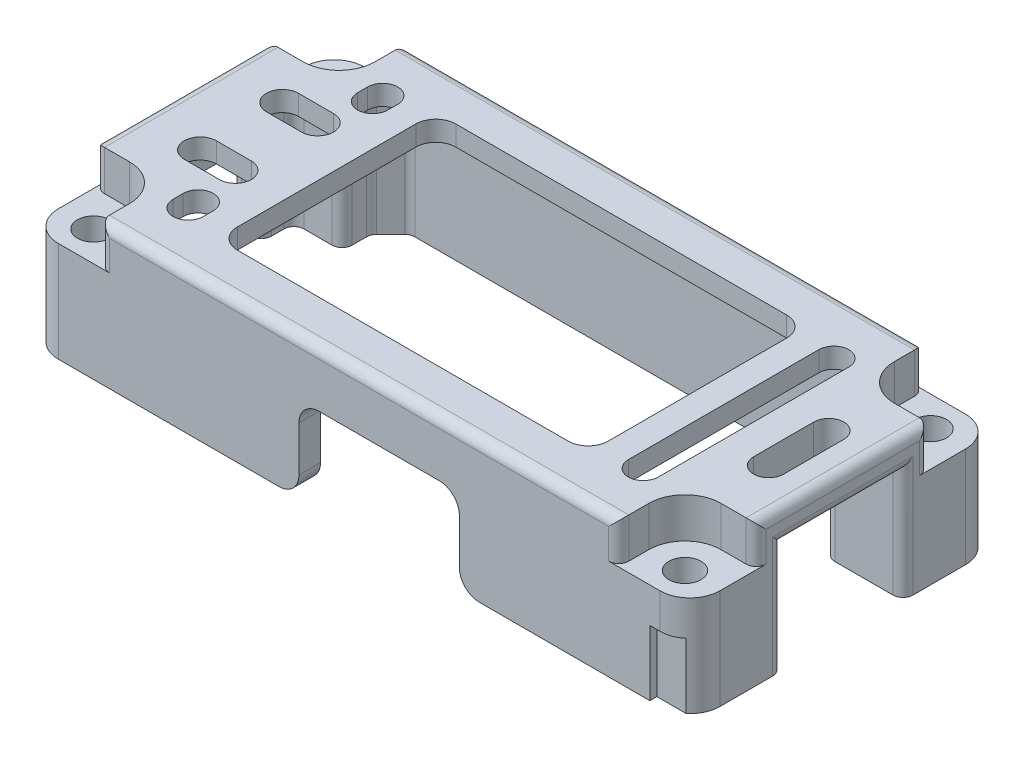
SolidWorks part; units mm, degrees
material "PUR"
ref_plane "前视基准面" through (0, 0, 0) normal (0, 0, 1) x (1, 0, 0)
ref_plane "上视基准面" through (0, 0, 0) normal (0, 1, 0) x (1, 0, 0)
ref_plane "右视基准面" through (0, 0, 0) normal (1, 0, 0) x (0, 0, -1)
sketch "草图1" plane through (0, 0, 0) normal (0, 1, 0) x (1, 0, 0)
  line L0 (-33, 4) -> (-27.6, 4)
  line L1 (-33, 15.25) -> (33, 15.25)
  line L2 (-33, 15.25) -> (-33, 4)
  line L3 (-33, -15.25) -> (33, -15.25)
  line L4 (33, 15.25) -> (33, 6)
  line L5 (-33, 15.25) -> (33, -15.25) construction
  line L6 (-33, -15.25) -> (33, 15.25) construction
  line L7 (-27.6, 4) -> (-27.6, -4)
  line L8 (-27.6, -4) -> (-33, -4)
  line L9 (-33, -4) -> (-33, -15.25)
  line L10 (33, 6) -> (28, 6)
  line L11 (28, 6) -> (28, -6)
  line L12 (28, -6) -> (33, -6)
  line L13 (33, -6) -> (33, -15.25)
  line L14 (-27.6, 0) -> (28, 0) construction
  line L15 (-26, -5.75) -> (-26, 5.75)
  line L16 (-26, 5.75) -> (-21.1, 5.75)
  line L17 (-21.1, 5.75) -> (-21.1, 13.1)
  line L18 (-21.1, 13.1) -> (21.1, 13.1)
  line L19 (21.1, 13.1) -> (21.1, -13.1)
  line L20 (21.1, -13.1) -> (-21.1, -13.1)
  line L21 (-21.1, -13.1) -> (-21.1, -5.75)
  line L22 (-21.1, -5.75) -> (-26, -5.75)
  line L23 (0, 15.25) -> (0, -15.25) construction
  circle A0 centre (-29.5, 12.25) radius 1.6
  circle A1 centre (29.5, 12.25) radius 1.6
  circle A2 centre (-29.5, -12.25) radius 1.6
  circle A3 centre (29.5, -12.25) radius 1.6
  point P0 (0, 0)
  dimension "D12" = 3.5
  dimension "D14" = 3.2
  dimension "D1" = 66
  dimension "D2" = 30.5
  dimension "D3" = 5.4
  dimension "D4" = 8
  dimension "D5" = 5
  dimension "D6" = 12
  dimension "D7" = 1.6
  dimension "D8" = 4.9
  dimension "D9" = 6.9
  dimension "D10" = 26.2
  dimension "D11" = 11.5
  dimension "D13" = 3
extrude "凸台-拉伸1" add sketch "草图1" along normal blind 12
sketch "草图2" plane through (0, 0, 0) normal (0, -1, 0) x (1, 0, 0)
  line L0 (21.1, -13.1) -> (-21.1, -13.1) construction
  line L1 (-21.1, 13.1) -> (21.1, 13.1) construction
  line L2 (26, -13.1) -> (-26, -13.1)
  line L3 (-26, 13.1) -> (26, 13.1)
  line L4 (-26, -5.75) -> (-26, 5.75) construction
  line L5 (-26, -13.1) -> (-26, 13.1)
  line L6 (26, 13.1) -> (26, -13.1)
  line L7 (28, 6) -> (28, -6) construction
  dimension "D1" = 2
extrude "切除-拉伸1" cut sketch "草图2" against normal blind 2
sketch "草图3" plane through (0, 12, 0) normal (0, 1, 0) x (1, 0, 0)
  line L0 (-26.8, 0) -> (21.1, 0) construction
  line L1 (-23.1, -10) -> (-30.5, -10)
  line L2 (-23.1, -10) -> (-23.1, 10)
  line L3 (-23.1, 10) -> (-30.5, 10)
  line L4 (-30.5, -10) -> (-30.5, 10)
  line L5 (-23.1, -10) -> (-30.5, 10) construction
  line L6 (-23.1, 10) -> (-30.5, -10) construction
  line L7 (-21.1, 13.1) -> (-21.1, 5.75) construction
  line L8 (28, -6) -> (28, 6) construction
  line L9 (28, -6) -> (28, 6)
  line L10 (21.1, 13.1) -> (21.1, -13.1)
  line L11 (26, 13.1) -> (21.1, 13.1)
  line L12 (26, -13.1) -> (26, 13.1)
  line L13 (21.1, -13.1) -> (26, -13.1)
  line L14 (21.1, 13.1) -> (21.1, -13.1)
  line L16 (26, -13.1) -> (26, -6)
  line L17 (21.1, -13.1) -> (26, -13.1)
  line L18 (28, 6) -> (26, 6)
  line L19 (28, -6) -> (26, -6)
  line L20 (26, 6) -> (26, 13.1)
  line L21 (21.1, 13.1) -> (-21.1, 13.1) construction
  line L22 (21.1, 13.1) -> (26, 13.1)
  point P0 (-26.8, 0)
  dimension "D1" = 20
  dimension "D2" = 0
  dimension "D3" = 7.4
  dimension "D4" = 2
extrude "切除-拉伸2" cut sketch "草图3" against normal blind 8
sketch "草图4" plane through (0, 0, 15.25) normal (0, 0, 1) x (1, 0, 0)
  line L1 (-6, 8.5) -> (10, 8.5)
  line L2 (-6, 8.5) -> (-6, 4)
  line L3 (-6, 4) -> (10, 4)
  line L4 (10, 8.5) -> (10, 4)
  line L5 (-33, 12) -> (33, 12) construction
  line L6 (33, 12) -> (33, 0) construction
  dimension "D1" = 16
  dimension "D2" = 23
  dimension "D3" = 3.5
  dimension "D4" = 4.5
extrude "切除-拉伸3" cut sketch "草图4" against normal up to surface (2.15 mm away) up to face at (5.2, 4, 13.1)
sketch "草图5" plane through (0, 0, 0) normal (0, -1, 0) x (1, 0, 0)
  line L0 (26, -13.1) -> (-26, -13.1) construction
  line L1 (26, -13.1) -> (26, 13.1) construction
  line L2 (-26, -13.1) -> (-26, 13.1) construction
  line L3 (-26, 13.1) -> (26, 13.1) construction
  line L4 (26, -13.1) -> (-26, -13.1)
  line L5 (26, -13.1) -> (26, 13.1)
  line L6 (-26, -13.1) -> (-26, 13.1)
  line L7 (-26, 13.1) -> (26, 13.1)
fillet "R1 圆角1" [suppressed] radius 1
fillet "R2 圆角2" [suppressed] radius 2
fillet "R3 圆角3" [suppressed] radius 3
extrude "切除-拉伸4" cut sketch "草图5" against normal through all
sketch "草图6" plane through (0, 12, 0) normal (0, 1, 0) x (1, 0, 0)
  line L4 (33, 6) -> (33, 15.25) construction
  line L5 (33, 15.25) -> (-33, 15.25) construction
  line L6 (-33, 15.25) -> (-33, 4) construction
  line L15 (-33, -15.25) -> (33, -15.25) construction
  line L24 (33, -15.25) -> (33, 15.25)
  line L25 (33, 15.25) -> (-33, 15.25)
  line L26 (-33, 15.25) -> (-33, -15.25)
  line L35 (-33, -15.25) -> (33, -15.25)
  line L40 (26, 13.1) -> (-26, 13.1) construction
  line L41 (-18.5, 10.9) -> (18.5, 10.9)
  line L42 (-18.5, 10.9) -> (-18.5, -10.9)
  line L44 (18.5, 10.9) -> (18.5, -10.9)
  line L45 (-33, 0) -> (33, 0) construction
  line L46 (-18.5, -10.9) -> (18.5, -10.9)
  line L47 (26, 6) -> (26, 13.1) construction
  line L48 (-26, 10) -> (-26, 13.1) construction
  circle A0 centre (-29.5, -12.25) radius 1.6 construction
  circle A1 centre (29.5, -12.25) radius 1.6 construction
  circle A2 centre (29.5, 12.25) radius 1.6 construction
  circle A3 centre (-29.5, 12.25) radius 1.6 construction
  circle A4 centre (-29.5, -12.25) radius 1.6
  circle A5 centre (29.5, -12.25) radius 1.6
  circle A6 centre (29.5, 12.25) radius 1.6
  circle A7 centre (-29.5, 12.25) radius 1.6
  dimension "D1" = 2.2
  dimension "D2" = 7.5
  dimension "D3" = 7.5
extrude "凸台-拉伸2" add sketch "草图6" along normal blind 2
sketch "草图7" plane through (0, 12, 0) normal (0, -1, 0) x (1, 0, 0)
  line L0 (28, 6) -> (28, -6) construction
  line L1 (26, -13.1) -> (26, 13.1) construction
  line L2 (-26, -13.1) -> (-26, 13.1) construction
  line L3 (-27.6, -4) -> (-27.6, 4) construction
  line L4 (28, 6) -> (28, -6)
  line L5 (26, -6) -> (26, 6)
  line L6 (-26, -4) -> (-26, 4)
  line L7 (-27.6, -4) -> (-27.6, 4)
  line L8 (-27.6, 4) -> (-26, 4)
  line L9 (-27.6, -4) -> (-26, -4)
  line L10 (28, 6) -> (26, 6)
  line L11 (28, -6) -> (26, -6)
extrude "切除-拉伸5" cut sketch "草图7" along normal through all
sketch "草图8" plane through (0, 8.5, 0) normal (0, -1, 0) x (1, 0, 0)
  line L4 (10, 13.1) -> (10, 15.25)
  line L5 (10, 15.25) -> (-6, 15.25)
  line L6 (-6, 15.25) -> (-6, 13.1)
  line L7 (-6, 13.1) -> (10, 13.1)
  line L8 (10, 13.1) -> (10, 15.25)
  line L9 (10, 15.25) -> (-6, 15.25)
  line L10 (-6, 15.25) -> (-6, 13.1)
  line L11 (-6, 13.1) -> (10, 13.1)
  dimension "D1" = 0
extrude "切除-拉伸6" cut sketch "草图8" along normal through all
sketch "草图9" plane through (0, 12, 0) normal (0, -1, 0) x (1, 0, 0)
  line L0 (25.2, 13.1) -> (26, 13.1)
  line L1 (-25.2, -13.1) -> (-26, -13.1)
  line L2 (-26, -10) -> (-30.5, -10) construction
  line L3 (-30.5, -10) -> (-30.5, -4) construction
  line L6 (-30.5, 4) -> (-30.5, 10) construction
  line L7 (-30.5, 10) -> (-26, 10) construction
  line L10 (-26, -10) -> (-30.5, -10)
  line L11 (-30.5, -10) -> (-30.5, -4)
  line L14 (-30.5, 4) -> (-30.5, 10)
  line L15 (-30.5, 10) -> (-26, 10)
  line L16 (-33, -4) -> (-30.5, -4) construction
  line L17 (-26, 4) -> (-33, 4) construction
  line L18 (-33, -4) -> (-33, 4) construction
  line L19 (-33, -4) -> (-30.5, -4)
  line L20 (-30.5, 4) -> (-33, 4)
  line L21 (-33, -4) -> (-33, 4)
  line L22 (-25.2, 13.1) -> (-25.2, -13.1)
  line L23 (-26, 13.1) -> (26, 13.1) construction
  line L24 (26, -13.1) -> (-26, -13.1) construction
  line L25 (-26, -10) -> (-26, -13.1) construction
  line L26 (-26, 4) -> (-26, 13.1) construction
  line L27 (26, -13.1) -> (25.2, -13.1)
  line L28 (-26, -10) -> (-26, -13.1)
  line L29 (-26, 10) -> (-26, 13.1)
  line L30 (-26, 13.1) -> (-25.2, 13.1)
  line L31 (26, -13.1) -> (26, -6) construction
  line L32 (26, 6) -> (26, 13.1) construction
  line L33 (26, -13.1) -> (26, -6)
  line L34 (26, 6) -> (26, 13.1)
  line L35 (25.2, 13.1) -> (25.2, 6)
  line L36 (25.2, 6) -> (26, 6)
  line L37 (25.2, -13.1) -> (25.2, -6)
  line L38 (25.2, -6) -> (26, -6)
  dimension "D1" = 0.8
  dimension "D2" = 0.8
extrude "凸台-拉伸3" add sketch "草图9" along normal through all
sketch "草图10" plane through (0, 0, 0) normal (0, -1, 0) x (1, 0, 0)
  line L1 (-33, -15.25) -> (-33, 15.25) construction
  line L3 (-33, -5) -> (-33, 5)
  line L4 (0, 0) -> (-25.2, 0) construction
  line L5 (-33, 5) -> (-30, 5)
  line L6 (-33, -5) -> (-30, -5)
  line L7 (-25.2, -13.1) -> (-25.2, 13.1) construction
  line L8 (-25.2, -8.25) -> (-25.2, 8.25)
  line L9 (-25.2, 8.25) -> (-30, 8.25)
  line L10 (-30, 8.25) -> (-30, 5)
  line L11 (-25.2, -8.25) -> (-30, -8.25)
  line L12 (-30, -8.25) -> (-30, -5)
  circle A0 centre (-29.5, 12.25) radius 1.6 construction
  dimension "D2" = 4
  dimension "D1" = 10
  dimension "D3" = 3
extrude "切除-拉伸7" cut sketch "草图10" against normal up to surface (12 mm away) up to face at (0, 12, 0)
sketch "草图11" plane through (0, 12, 0) normal (0, -1, 0) x (1, 0, 0)
  line L0 (-33, -5) -> (-30, -5) construction
  line L1 (-30, 5) -> (-33, 5) construction
  line L2 (-33, 5) -> (-33, -5) construction
  line L3 (-33, -5) -> (-30, -5)
  line L4 (-30, 5) -> (-33, 5)
  line L5 (-33, 5) -> (-33, -5)
  line L6 (-30, 5) -> (-30, -5)
extrude "凸台-拉伸4" add sketch "草图11" along normal blind 3
sketch "草图13" plane through (0, 12, 0) normal (0, -1, 0) x (1, 0, 0)
  line L0 (25.2, -6) -> (33, -6) construction
  line L1 (33, 6) -> (33, -6) construction
  line L2 (33, 6) -> (25.2, 6) construction
  line L3 (25.2, -6) -> (33, -6)
  line L4 (33, 6) -> (33, -6)
  line L5 (33, 6) -> (25.2, 6)
  line L6 (25.2, 6) -> (25.2, -6)
extrude "凸台-拉伸5" add sketch "草图13" along normal blind 1
chamfer "倒角1" distance 2 angle 45 4 edges at (-25.2, 6, -13.1) (25.2, 6, -13.1) (25.2, 6, 13.1) (-25.2, 6, 13.1)
sketch "草图12" plane through (0, 14, 0) normal (0, 1, 0) x (1, 0, 0)
  line L0 (-29.5, 8.65) -> (-33, 8.65)
  line L1 (-33, 15.25) -> (-33, -15.25) construction
  line L2 (-25.9, 12.25) -> (-25.9, 15.25)
  line L3 (33, 15.25) -> (-33, 15.25) construction
  line L4 (29.5, 8.65) -> (33, 8.65)
  line L5 (33, -15.25) -> (33, 15.25) construction
  line L6 (25.9, 12.25) -> (25.9, 15.25)
  line L7 (29.5, -8.65) -> (33, -8.65)
  line L8 (25.9, -12.25) -> (25.9, -15.25)
  line L9 (-33, -15.25) -> (33, -15.25) construction
  line L10 (-25.9, -12.25) -> (-25.9, -15.25)
  line L11 (-29.5, -8.65) -> (-33, -8.65)
  line L12 (-33, -8.65) -> (-33, -15.25)
  line L13 (-25.9, 15.25) -> (-33, 15.25)
  line L14 (33, 8.65) -> (33, 15.25)
  line L15 (25.9, -15.25) -> (33, -15.25)
  line L16 (33, 15.25) -> (-33, 15.25)
  line L17 (-33, 15.25) -> (-33, -15.25)
  line L18 (-33, -15.25) -> (33, -15.25)
  line L19 (33, -15.25) -> (33, 15.25)
  line L20 (33, 15.25) -> (25.9, 15.25)
  line L21 (-33, 15.25) -> (-33, 8.65)
  line L22 (-33, -15.25) -> (-25.9, -15.25)
  line L23 (33, -15.25) -> (33, -8.65)
  arc A0 (-29.5, 8.65) -> (-25.9, 12.25) centre (-29.5, 12.25) ccw
  arc A1 (25.9, 12.25) -> (29.5, 8.65) centre (29.5, 12.25) ccw
  arc A2 (29.5, -8.65) -> (25.9, -12.25) centre (29.5, -12.25) ccw
  arc A3 (-25.9, -12.25) -> (-29.5, -8.65) centre (-29.5, -12.25) ccw
  dimension "D1" = 7.2
  dimension "D2" = 0
extrude "切除-拉伸8" cut sketch "草图12" against normal blind 4
sketch "草图14" plane through (0, 14, 0) normal (0, 1, 0) x (1, 0, 0)
  line L0 (-33, 0) -> (33, 0) construction
  line L1 (-33, 8.65) -> (-33, -8.65) construction
  line L2 (33, -8.65) -> (33, 8.65) construction
  line L3 (22.6, -9.5) -> (22.6, 9.5) construction
  line L4 (21.1, -9.5) -> (21.1, 9.5)
  line L5 (24.1, -9.5) -> (24.1, 9.5)
  line L6 (28.6, -3) -> (28.6, 3) construction
  line L7 (27.1, -3) -> (27.1, 3)
  line L8 (30.1, -3) -> (30.1, 3)
  line L9 (18.5, -10.9) -> (18.5, 10.9) construction
  line L10 (-27, 4.1) -> (-23.5, 4.1) construction
  line L11 (-27, 5.7) -> (-23.5, 5.7)
  line L12 (-27, 2.5) -> (-23.5, 2.5)
  line L13 (-27, -4.1) -> (-23.5, -4.1) construction
  line L14 (-27, -5.7) -> (-23.5, -5.7)
  line L15 (-27, -2.5) -> (-23.5, -2.5)
  line L16 (-18.5, 10.9) -> (-18.5, -10.9) construction
  line L17 (-22.6, 9.7) -> (-22.6, 8.7) construction
  line L18 (-21.1, 9.7) -> (-21.1, 8.7)
  line L19 (-24.1, 9.7) -> (-24.1, 8.7)
  line L20 (-22.6, -9.7) -> (-22.6, -8.7) construction
  line L21 (-21.1, -9.7) -> (-21.1, -8.7)
  line L22 (-24.1, -9.7) -> (-24.1, -8.7)
  arc A0 (21.1, -9.5) -> (24.1, -9.5) centre (22.6, -9.5) ccw
  arc A1 (24.1, 9.5) -> (21.1, 9.5) centre (22.6, 9.5) ccw
  arc A2 (27.1, -3) -> (30.1, -3) centre (28.6, -3) ccw
  arc A3 (30.1, 3) -> (27.1, 3) centre (28.6, 3) ccw
  arc A4 (-27, 5.7) -> (-27, 2.5) centre (-27, 4.1) ccw
  arc A5 (-23.5, 2.5) -> (-23.5, 5.7) centre (-23.5, 4.1) ccw
  arc A6 (-27, -5.7) -> (-27, -2.5) centre (-27, -4.1) cw
  arc A7 (-23.5, -2.5) -> (-23.5, -5.7) centre (-23.5, -4.1) cw
  arc A8 (-21.1, 9.7) -> (-24.1, 9.7) centre (-22.6, 9.7) ccw
  arc A9 (-24.1, 8.7) -> (-21.1, 8.7) centre (-22.6, 8.7) ccw
  arc A10 (-21.1, -9.7) -> (-24.1, -9.7) centre (-22.6, -9.7) cw
  arc A11 (-24.1, -8.7) -> (-21.1, -8.7) centre (-22.6, -8.7) cw
  point P8 (22.6, 0)
  point P14 (28.6, 0)
  point P23 (-25.25, 4.1)
  point P31 (-25.25, -4.1)
  point P40 (-22.6, 9.2)
  point P47 (-22.6, -9.2)
  dimension "D1" = 3
  dimension "D9" = 1.6
  dimension "D2" = 2.6
  dimension "D3" = 19
  dimension "D4" = 3
  dimension "D5" = 6
  dimension "D6" = 6
  dimension "D7" = 5
  dimension "D8" = 5
  dimension "D10" = 2.6
  dimension "D11" = 3
  dimension "D12" = 1
extrude "切除-拉伸9" cut sketch "草图14" against normal through all
fillet "R1 过渡圆角" radius 1 34 edges at (-33, 4.5, 5) (-33, 4.5, -5) (-30, 4.5, 5) (-30, 4.5, -5) (33, 5.5, 6) (33, 5.5, -6) (25.2, 5.5, -6) (25.2, 5.5, 6) (25.2, 6, 11.1) (23.2, 6, 13.1) (-23.2, 6, 13.1) (-25.2, 6, 11.1) (-25.2, 6, 8.25) (-30, 6, 8.25) (-30, 6, -8.25) (-25.2, 6, -8.25) (-25.2, 6, -11.1) (-23.2, 6, -13.1) (23.2, 6, -13.1) (25.2, 6, -11.1) (33, 12, 8.65) (25.9, 12, 15.25) (25.9, 12, -15.25) (33, 12, -8.65) (-25.9, 12, -15.25) (-33, 12, -8.65) (-25.9, 12, 15.25) (-33, 12, 8.65) (33, 14, 0) (0, 14, 15.25) (-33, 14, 0) (0, 14, -15.25) (33, 11, 0) (-33, 9, 0)
fillet "R2 过渡圆角" radius 2 8 edges at (10, 8.5, 14.175) (-6, 8.5, 14.175) (-18.5, 13, 10.9) (18.5, 13, 10.9) (18.5, 13, -10.9) (-18.5, 13, -10.9) (10, 0, 14.175) (-6, 0, 14.175)
fillet "R3 过渡圆角" radius 3 4 edges at (33, 5, 15.25) (-33, 5, 15.25) (-33, 5, -15.25) (33, 5, -15.25)
sketch "草图15" plane through (0, 0, 0) normal (0, -1, 0) x (1, 0, 0)
  line L0 (12, 15.25) -> (30, 15.25) construction
  line L1 (29, 15.25) -> (30, 15.25)
  line L2 (31.9261, 14.55) -> (29, 14.55)
  line L3 (29, 14.55) -> (29, 15.25)
  line L4 (33, 12.25) -> (33, 7) construction
  arc A0 (33, 12.25) -> (30, 15.25) centre (30, 12.25) ccw construction
  arc A1 (31.9261, 14.55) -> (30, 15.25) centre (30, 12.25) ccw
  dimension "D1" = 0.7
  dimension "D2" = 4
extrude "切除-拉伸10" cut sketch "草图15" against normal blind 6.5
